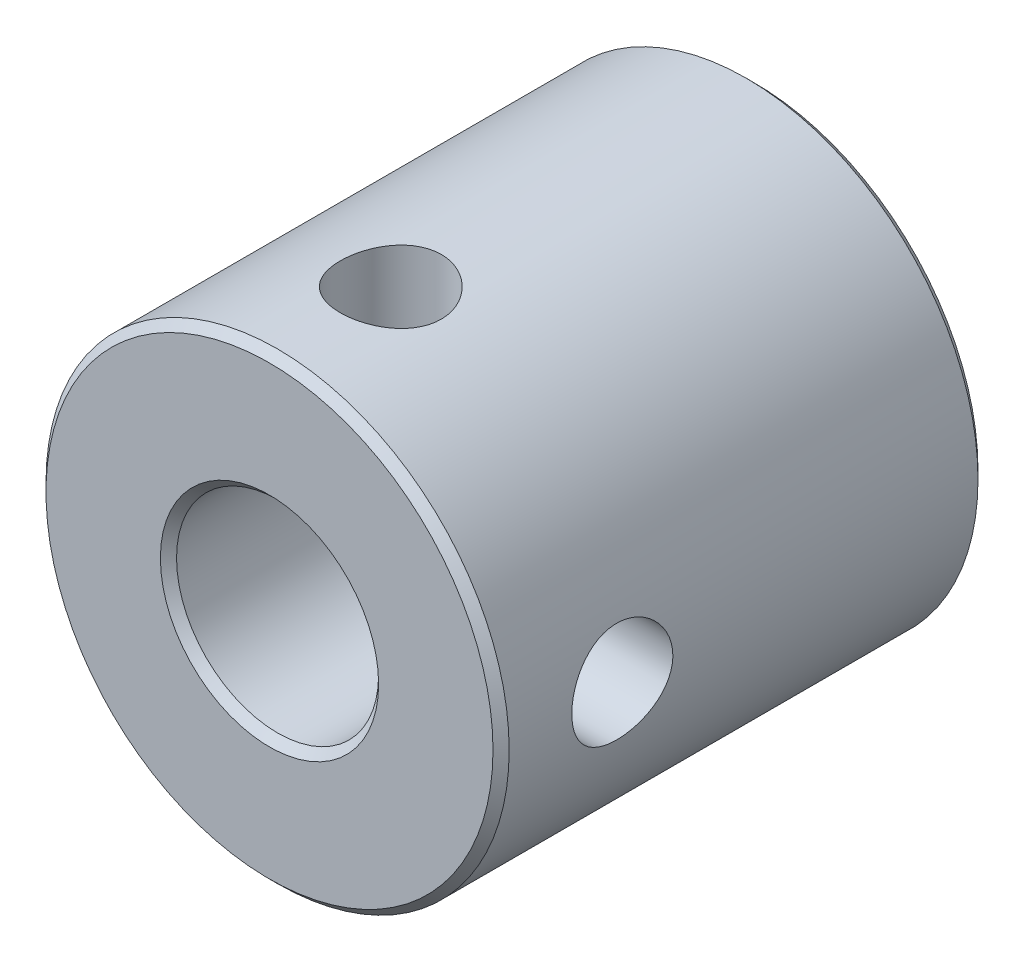
from build123d import *

# Parameters (mm, degrees)
SKETCH3_W = 1.25
SKETCH3_H = 5.73
SKETCH5_W = 1.25
SKETCH5_H = 5.73


with BuildPart() as part:
    # Sketch1 → Revolve1 (revolve)
    with BuildSketch(Plane(origin=(0, 0, 0), x_dir=(1, 0, 0), z_dir=(0, 1, 0))):
        Polygon((2.7, 0), (5.53, 0), (5.73, 0.2), (5.73, 11.8), (5.53, 12), (2.7, 12), (2.5, 11.8), (2.5, 0.2), align=None)
    revolve(axis=Axis((0, 0, 0), (0, 0, -1)))

    # Sketch3 → M3 Tapped Hole1 (revolve, cut)
    with BuildSketch(Plane(origin=(0, 0, -3), x_dir=(0, 0, -1), z_dir=(1, 0, 0))):
        with Locations((0.625, 2.865)):
            Rectangle(SKETCH3_W, SKETCH3_H)
    revolve(axis=Axis((0, -6.35, -3), (0, 1, 0)), mode=Mode.SUBTRACT)

    # Sketch5 → M3 Tapped Hole2 (revolve, cut)
    with BuildSketch(Plane(origin=(0, 0, -3), x_dir=(0, 0, 1), z_dir=(0, 1, 0))):
        with Locations((0.625, 2.865)):
            Rectangle(SKETCH5_W, SKETCH5_H)
    revolve(axis=Axis((-6.35, 0, -3), (1, 0, 0)), mode=Mode.SUBTRACT)


solid = part.part
